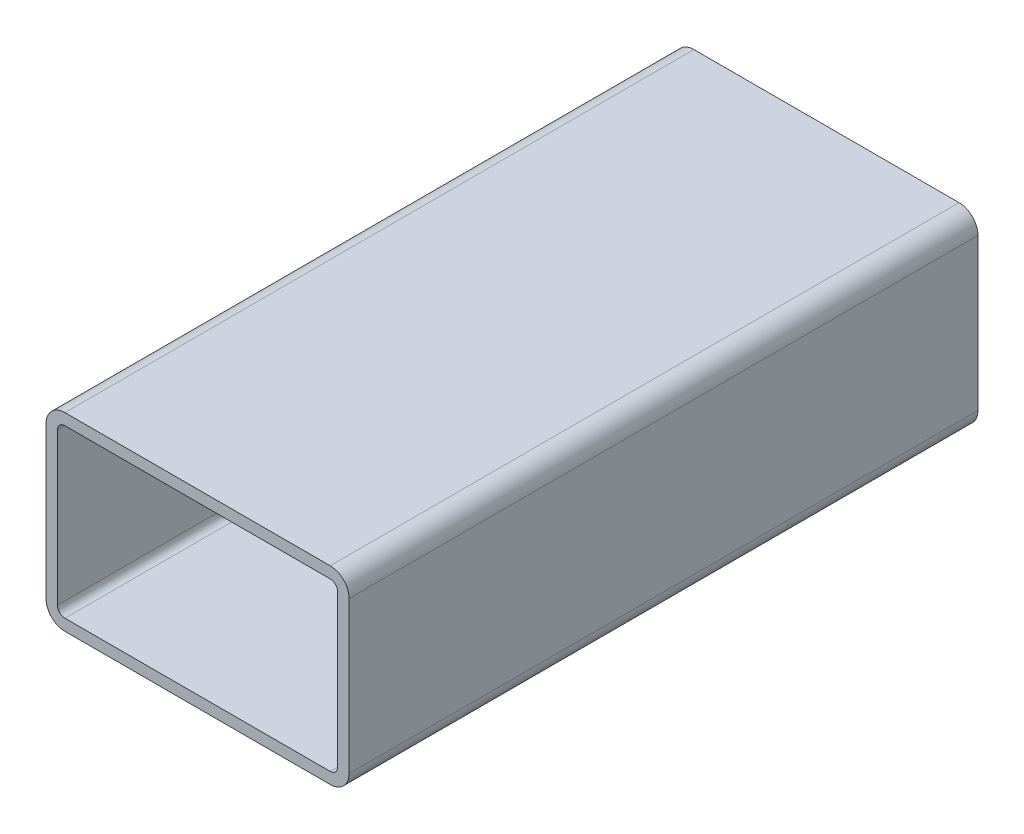
from build123d import *

# Parameters (mm, degrees)
SKETCH1_W           = 80
SKETCH1_H           = 50
BOSS_EXTRUDE1_DEPTH = 166
FILLET1_R           = 5
SHELL1_T            = -3


with BuildPart() as part:
    # Sketch1 → Boss-Extrude1 (new body)
    with BuildSketch(Plane.XY):
        Rectangle(SKETCH1_W, SKETCH1_H)
    extrude(amount=BOSS_EXTRUDE1_DEPTH)

    # Fillet1
    fillet1_edges = [part.edges().sort_by_distance(p)[0] for p in [
        (-40, 25, 83),
        (40, 25, 83),
        (40, -25, 83),
        (-40, -25, 83),
    ]]
    fillet(fillet1_edges, radius=FILLET1_R)

    # Shell1
    shell1_openings = [part.faces().sort_by_distance(p)[0] for p in [
        (0, 0, 166),
        (0, 0, 0),
    ]]
    offset(amount=SHELL1_T, openings=shell1_openings, kind=Kind.INTERSECTION)


solid = part.part
